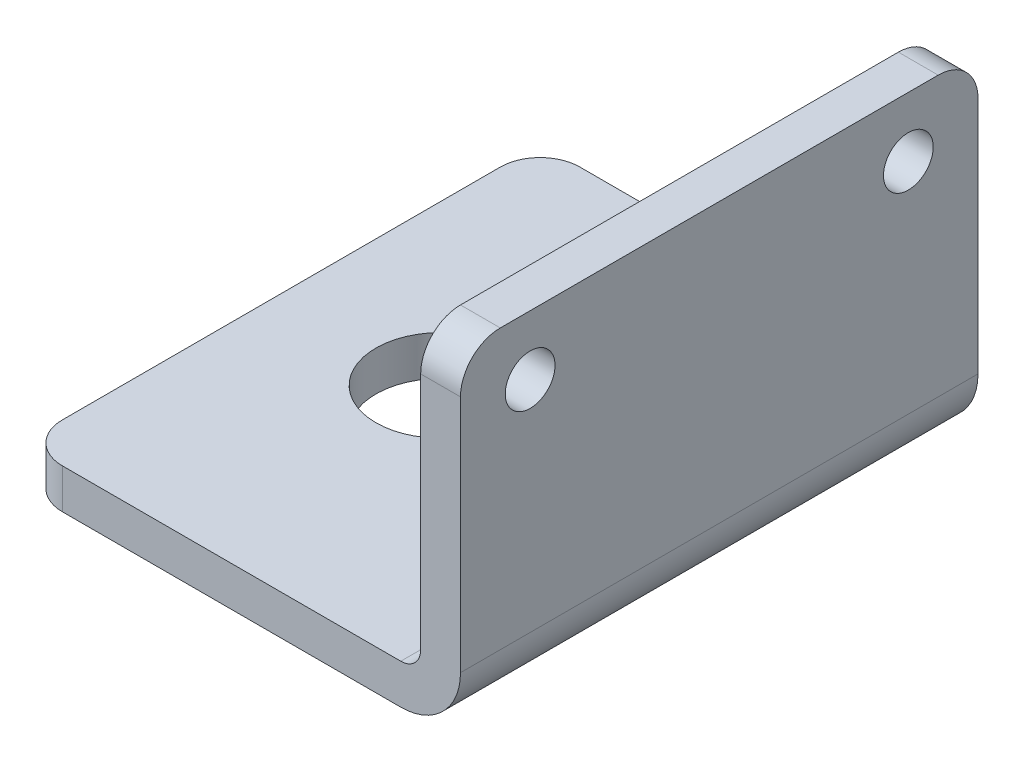
from build123d import *

# Parameters (mm, degrees)
EXTRUDE_1_DEPTH     = 26
FILLET_1_R          = 1
FILLET_2_R          = 3
FILLET_3_R          = 2
SKETCH_2_R          = 3.25
CUT_EXTRUDE_1_DEPTH = 38.215588132
HOLE_WIZARD_M3_1_D  = 2.5


with BuildPart() as part:
    # 草图1 → 拉伸-薄壁1 (new body)
    with BuildSketch(Plane.XY):
        Polygon((0, 0), (20, 0), (20, 15), (22, 15), (22, -2), (0, -2), align=None)
    extrude(amount=EXTRUDE_1_DEPTH)

    # 圆角1
    fillet_1_edges = [part.edges().sort_by_distance(p)[0] for p in [
        (20, 0, 13),
    ]]
    fillet(fillet_1_edges, radius=FILLET_1_R)

    # 圆角2
    fillet_2_edges = [part.edges().sort_by_distance(p)[0] for p in [
        (22, -2, 13),
    ]]
    fillet(fillet_2_edges, radius=FILLET_2_R)

    # 圆角3
    fillet_3_edges = [part.edges().sort_by_distance(p)[0] for p in [
        (0, -1, 26),
        (0, -1, 0),
        (21, 15, 0),
        (21, 15, 26),
    ]]
    fillet(fillet_3_edges, radius=FILLET_3_R)

    # 草图2 → 切除-拉伸1 (cut, through all)
    with BuildSketch(Plane(origin=(0, 0, 0), x_dir=(1, 0, 0), z_dir=(0, 1, 0))):
        with Locations(Location((8, -13, 0), (0, 0, 270))):
            Circle(SKETCH_2_R)
    extrude(amount=-CUT_EXTRUDE_1_DEPTH, mode=Mode.SUBTRACT)

    # M3 螺纹孔1 (through all)
    with Locations(Plane(origin=(22, 0, 0), x_dir=(0, 0, -1), z_dir=(1, 0, 0))):
        with Locations((-22.5, 12), (-3.5, 12)):
            Hole(HOLE_WIZARD_M3_1_D / 2)


solid = part.part
